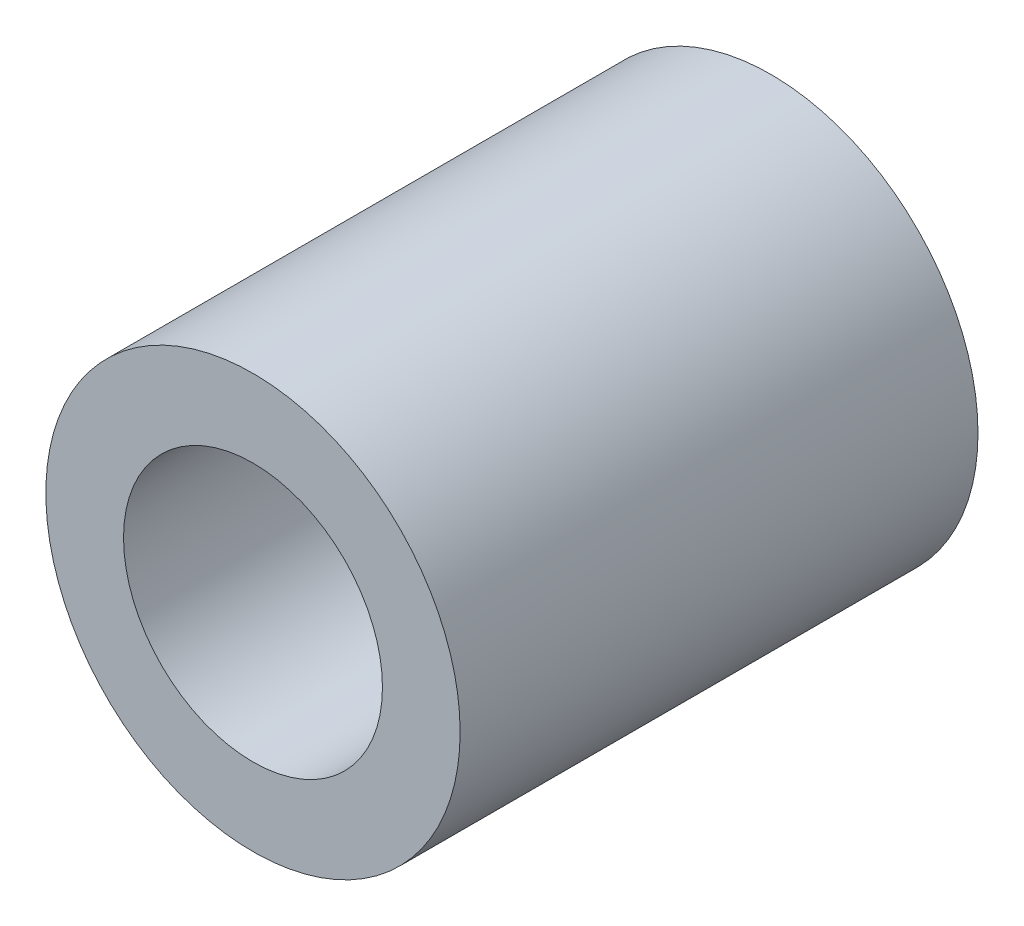
from build123d import *

# Parameters (mm, degrees)
SKETCH_1_R      = 20
SKETCH_1_R_2    = 12.5
EXTRUDE_1_DEPTH = 25


with BuildPart() as part:
    # 草图1 → 凸台-拉伸1 (new, symmetric)
    with BuildSketch(Plane.XY):
        Circle(SKETCH_1_R)
        Circle(SKETCH_1_R_2, mode=Mode.SUBTRACT)
    extrude(amount=EXTRUDE_1_DEPTH, both=True)


solid = part.part
